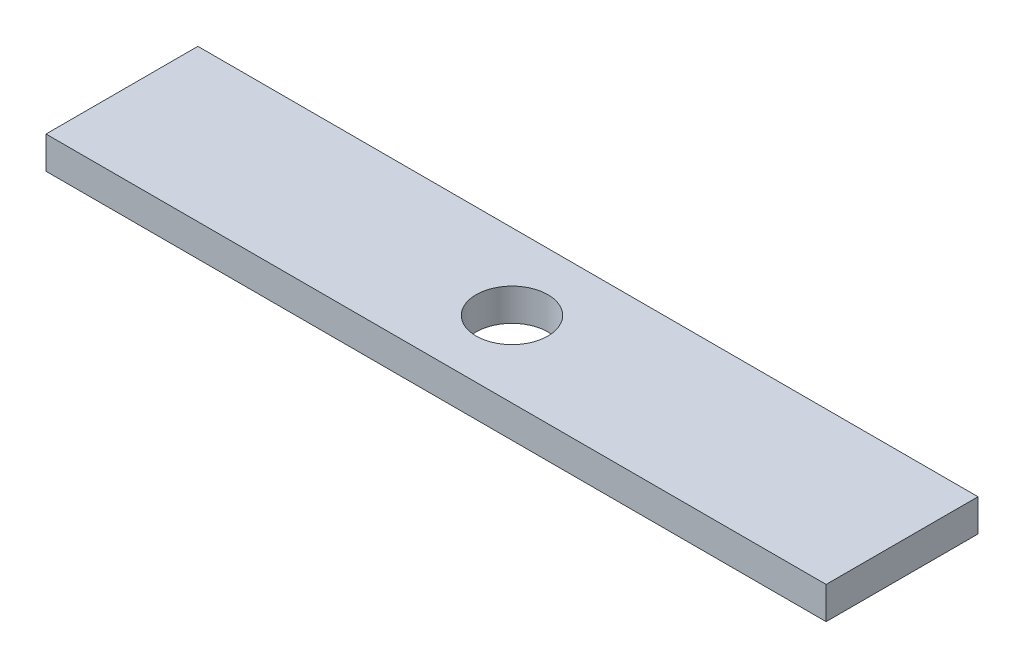
from build123d import *

# Parameters (mm, degrees)
SKETCH1_W           = 108.732266051
SKETCH1_H           = 21.168090093
SKETCH1_R           = 5
BOSS_EXTRUDE1_DEPTH = 4.5


with BuildPart() as part:
    # Sketch1 → Boss-Extrude1 (new body)
    with BuildSketch(Plane(origin=(0, 0, 0), x_dir=(1, 0, 0), z_dir=(0, 1, 0))):
        with Locations((54.366133026, 10.584045046)):
            Rectangle(SKETCH1_W, SKETCH1_H)
        with Locations(Location((54.366133025, 10.584045046, 0), (0, 0, 270))):
            Circle(SKETCH1_R, mode=Mode.SUBTRACT)
    extrude(amount=BOSS_EXTRUDE1_DEPTH)


solid = part.part
